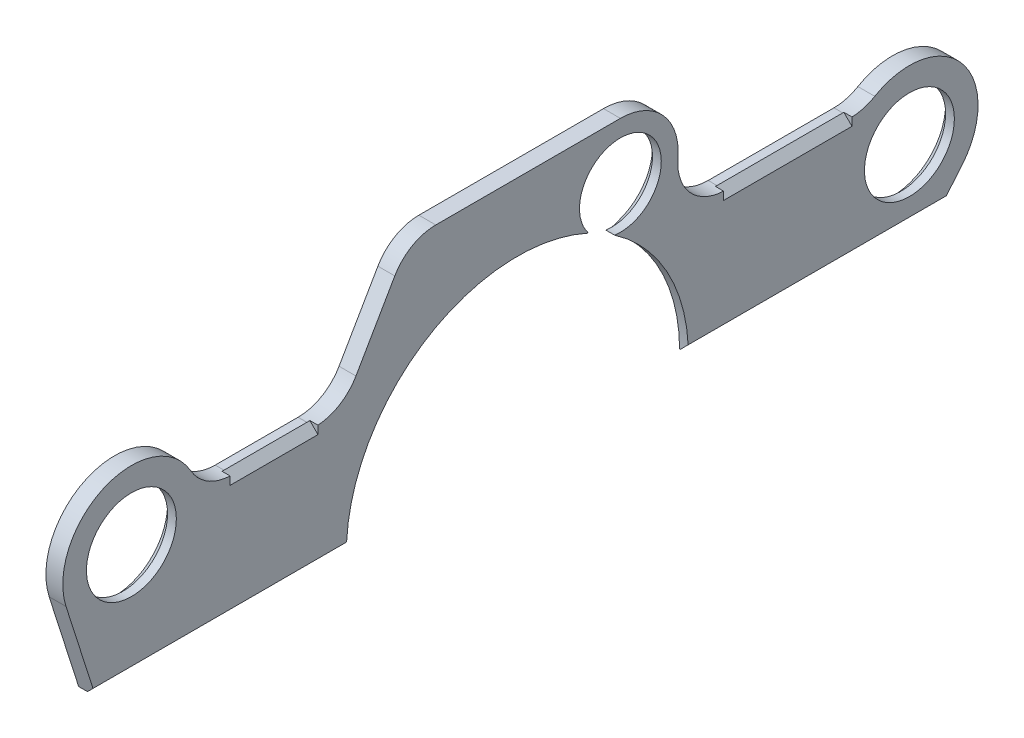
from build123d import *

# Parameters (mm, degrees)
BOSS_EXTRUDE1_DEPTH     = 12.5
CUT_EXTRUDE1_DEPTH      = 768.828594154
CUT_EXTRUDE1_DEPTH_BACK = 768.828594154
SKETCH2_R               = 60.5
SKETCH2_R_2             = 66.5
FILLET1_R               = 70
CHAMFER1_SIZE           = 12
CHAMFER2_SIZE           = 12
CUT_EXTRUDE2_DEPTH      = 65
CUT_EXTRUDE3_DEPTH      = 95


with BuildPart() as part:
    # Sketch1 → Boss-Extrude1 (new, symmetric)
    with BuildSketch(Plane(origin=(0, 0, 0), x_dir=(0, 0, -1), z_dir=(1, 0, 0))):
        with BuildLine():
            Line((-161.139129372, 353.5), (152.4, 353.5))
            ThreePointArc((152.4, 353.5), (215.520549571, 325.671884154), (237.552772458, 260.302250804))
            ThreePointArc((237.552772458, 260.302250804), (255.590849676, 206.783252739), (307.268492599, 184))
            Line((307.268492599, 184), (515.051943832, 184))
            ThreePointArc((515.051943832, 184), (651.90709321, 177.635326105), (657.753510977, 40.757057617))
            Line((657.753510977, 40.757057617), (624.56119852, 1.2))
            Line((624.56119852, 1.2), (252.997154134, 1.2))
            ThreePointArc((252.997154134, 1.2), (0, 253), (-252.997154134, 1.2))
            Line((-252.997154134, 1.2), (-624, 1.2))
            Line((-624, 1.2), (-667.696816027, 138.145895408))
            ThreePointArc((-667.696816027, 138.145895408), (-594.001115997, 267.859489493), (-470.614493078, 184))
            Line((-470.614493078, 184), (-259, 184))
            Line((-259, 184), (-161.139129372, 353.5))
        make_face()
    extrude(amount=BOSS_EXTRUDE1_DEPTH, both=True)

    # Sketch2 → Cut-Extrude1 (cut, two sides: drawn at the far end of the back side and taken through both)
    with BuildSketch(Plane(origin=(0, 0, 0), x_dir=(0, 0, -1), z_dir=(1, 0, 0)).offset(-CUT_EXTRUDE1_DEPTH_BACK)):
        with Locations((152.4, 268)):
            Circle(SKETCH2_R)
        with Locations((-571, 169)):
            Circle(SKETCH2_R_2)
        with Locations((580, 106)):
            Circle(SKETCH2_R_2)
    extrude(amount=CUT_EXTRUDE1_DEPTH + CUT_EXTRUDE1_DEPTH_BACK, mode=Mode.SUBTRACT)

    # Fillet1
    fillet1_edges = [part.edges().sort_by_distance(p)[0] for p in [
        (0, 184, 470.614493078),
        (0, 184, 259),
        (0, 353.5, 161.139129372),
        (0, 184, -515.051943832),
    ]]
    fillet(fillet1_edges, radius=FILLET1_R)

    # Chamfer1
    chamfer1_edges = [part.edges().sort_by_distance(p)[0] for p in [
        (12.5, 1.2, 438.498577067),
        (12.5, 1.2, -438.779176327),
    ]]
    chamfer(chamfer1_edges, length=CHAMFER1_SIZE)

    # Chamfer2
    chamfer2_edges = [part.edges().sort_by_distance(p)[0] for p in [
        (-12.5, 213.213707904, 136.194400626),
        (-12.5, 118.018425376, -223.787066811),
        (-12.5, 320.591390839, -182.306447626),
        (-12.5, 169, 637.5),
        (-12.5, 106, -513.5),
    ]]
    chamfer(chamfer2_edges, length=CHAMFER2_SIZE)

    # Sketch3 → Cut-Extrude2 (cut, symmetric)
    with BuildSketch(Plane.XY.offset(360)):
        Polygon((-5.5, 190), (12.5, 172), (12.5, 190), align=None)
    extrude(amount=CUT_EXTRUDE2_DEPTH, both=True, mode=Mode.SUBTRACT)

    # Sketch4 → Cut-Extrude3 (cut, symmetric)
    with BuildSketch(Plane.XY.offset(-400)):
        Polygon((12.5, 190), (-5.5, 190), (12.5, 172), align=None)
    extrude(amount=CUT_EXTRUDE3_DEPTH, both=True, mode=Mode.SUBTRACT)


solid = part.part
